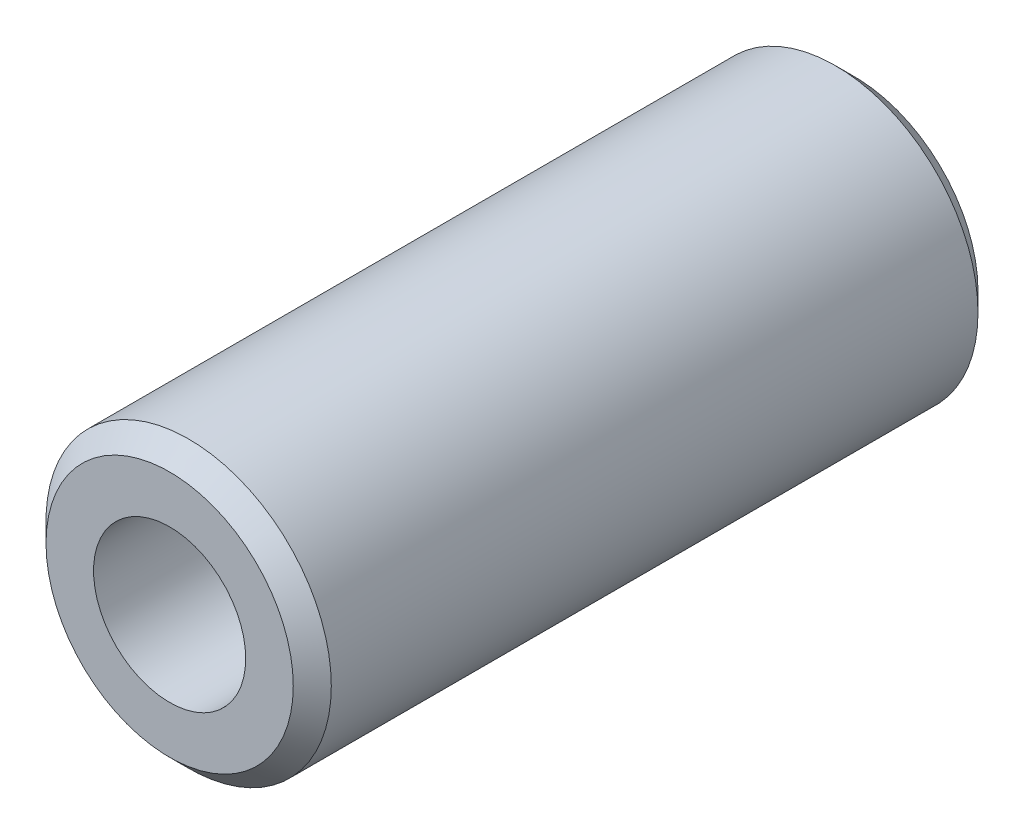
SolidWorks part; units mm, degrees
ref_plane "Front Plane" through (0, 0, 0) normal (0, 0, 1) x (1, 0, 0)
ref_plane "Top Plane" through (0, 0, 0) normal (0, 1, 0) x (1, 0, 0)
ref_plane "Right Plane" through (0, 0, 0) normal (1, 0, 0) x (0, 0, -1)
sketch "Sketch1" plane through (0, 0, 0) normal (0, 0, 1) x (1, 0, 0)
  circle A0 centre (0, 0) radius 7.5
  dimension "D1" = 15
extrude "Boss-Extrude1" add sketch "Sketch1" along normal blind 36
chamfer "Chamfer1" distance 1 angle 45 2 edges at (7.5, 0, 0) (7.5, 0, 36)
sketch "Sketch2" plane through (0, 0, 36) normal (0, 0, 1) x (1, 0, 0)
  circle A0 centre (0, 0) radius 4
  dimension "D1" = 8
extrude "Cut-Extrude1" cut sketch "Sketch2" against normal through all
